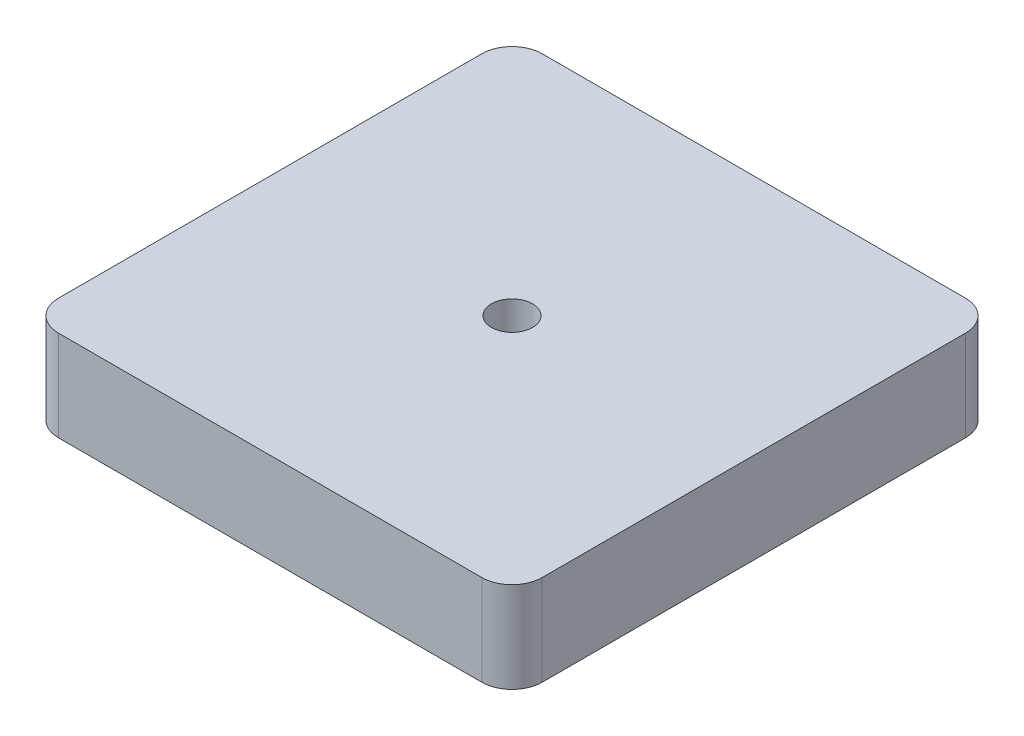
from build123d import *

# Parameters (mm, degrees)
SKETCH_1_W             = 80
SKETCH_1_H             = 80
EXTRUDE_1_DEPTH        = 15
FILLET_1_R             = 5
HOLE_WIZARD_M8_1_D     = 6.8
HOLE_WIZARD_M8_1_DEPTH = 19.75
HOLE_WIZARD_M8_1_TIP   = 2.042926105


with BuildPart() as part:
    # 草图1 → 凸台-拉伸1 (new body)
    with BuildSketch(Plane(origin=(0, 0, 0), x_dir=(1, 0, 0), z_dir=(0, 1, 0))):
        Rectangle(SKETCH_1_W, SKETCH_1_H)
    extrude(amount=EXTRUDE_1_DEPTH)

    # 圆角1
    fillet_1_edges = [part.edges().sort_by_distance(p)[0] for p in [
        (40, 7.5, 40),
        (-40, 7.5, 40),
        (-40, 7.5, -40),
        (40, 7.5, -40),
    ]]
    fillet(fillet_1_edges, radius=FILLET_1_R)

    # M8 螺纹孔1
    with Locations(Plane(origin=(0, 0, 0), x_dir=(-1, 0, 0), z_dir=(0, -1, 0))):
        with Locations((0, 0)):
            Hole(HOLE_WIZARD_M8_1_D / 2, depth=HOLE_WIZARD_M8_1_DEPTH)
            with Locations((0, 0, -(HOLE_WIZARD_M8_1_DEPTH + HOLE_WIZARD_M8_1_TIP / 2))):  # 118° drill point
                Cone(0, HOLE_WIZARD_M8_1_D / 2, HOLE_WIZARD_M8_1_TIP, mode=Mode.SUBTRACT)


solid = part.part
